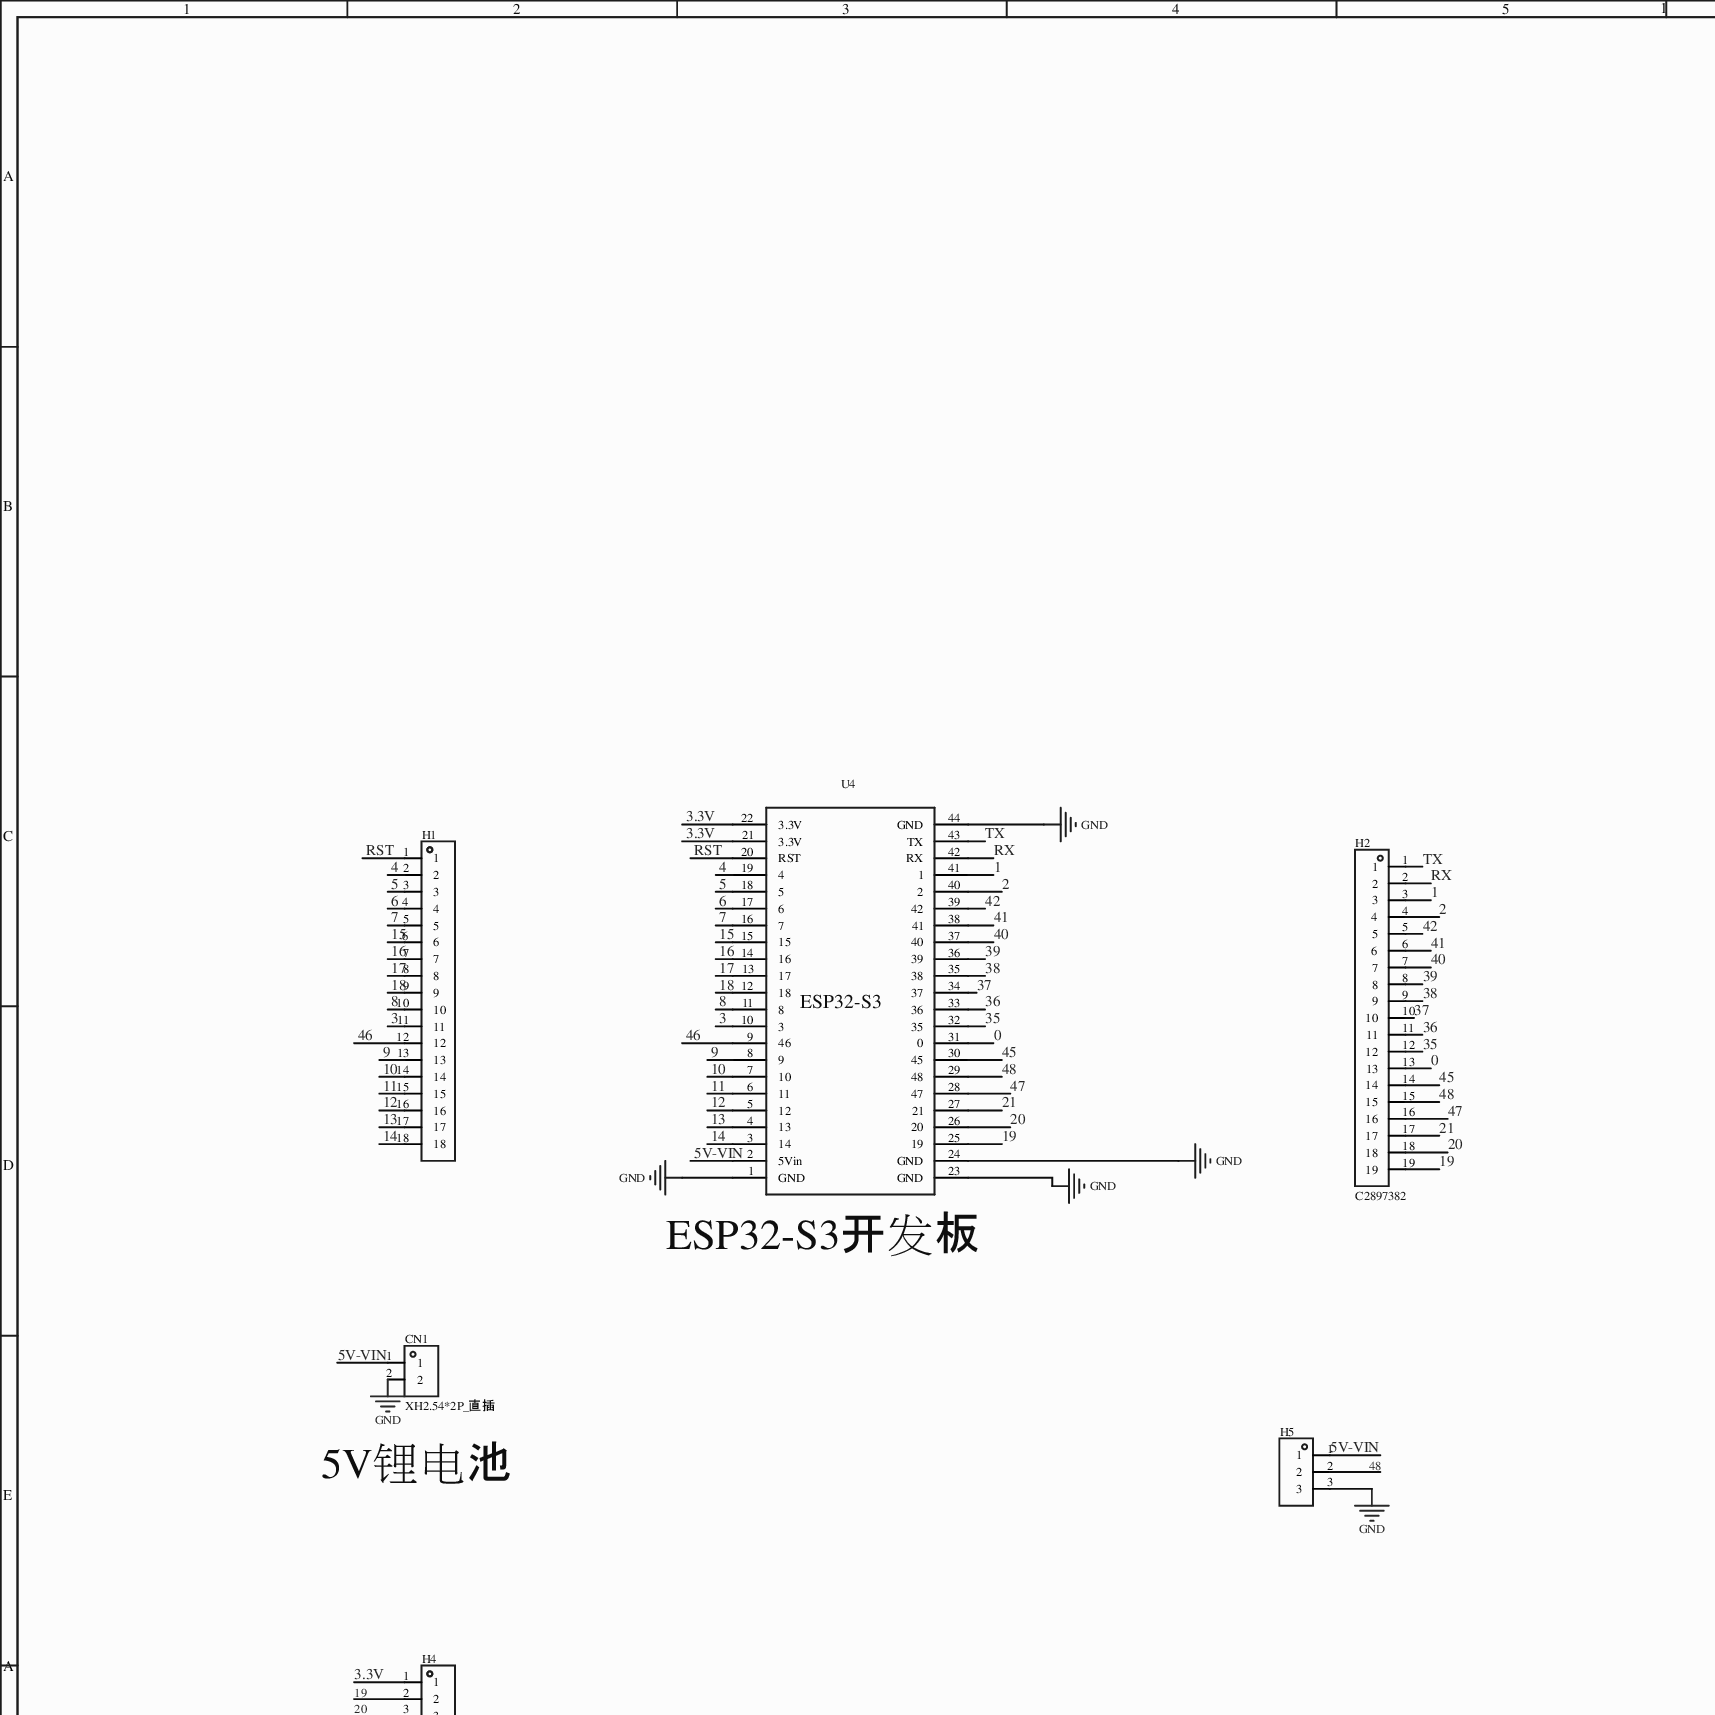
[diagram p0: MISC52029-3.schdoc, top left]
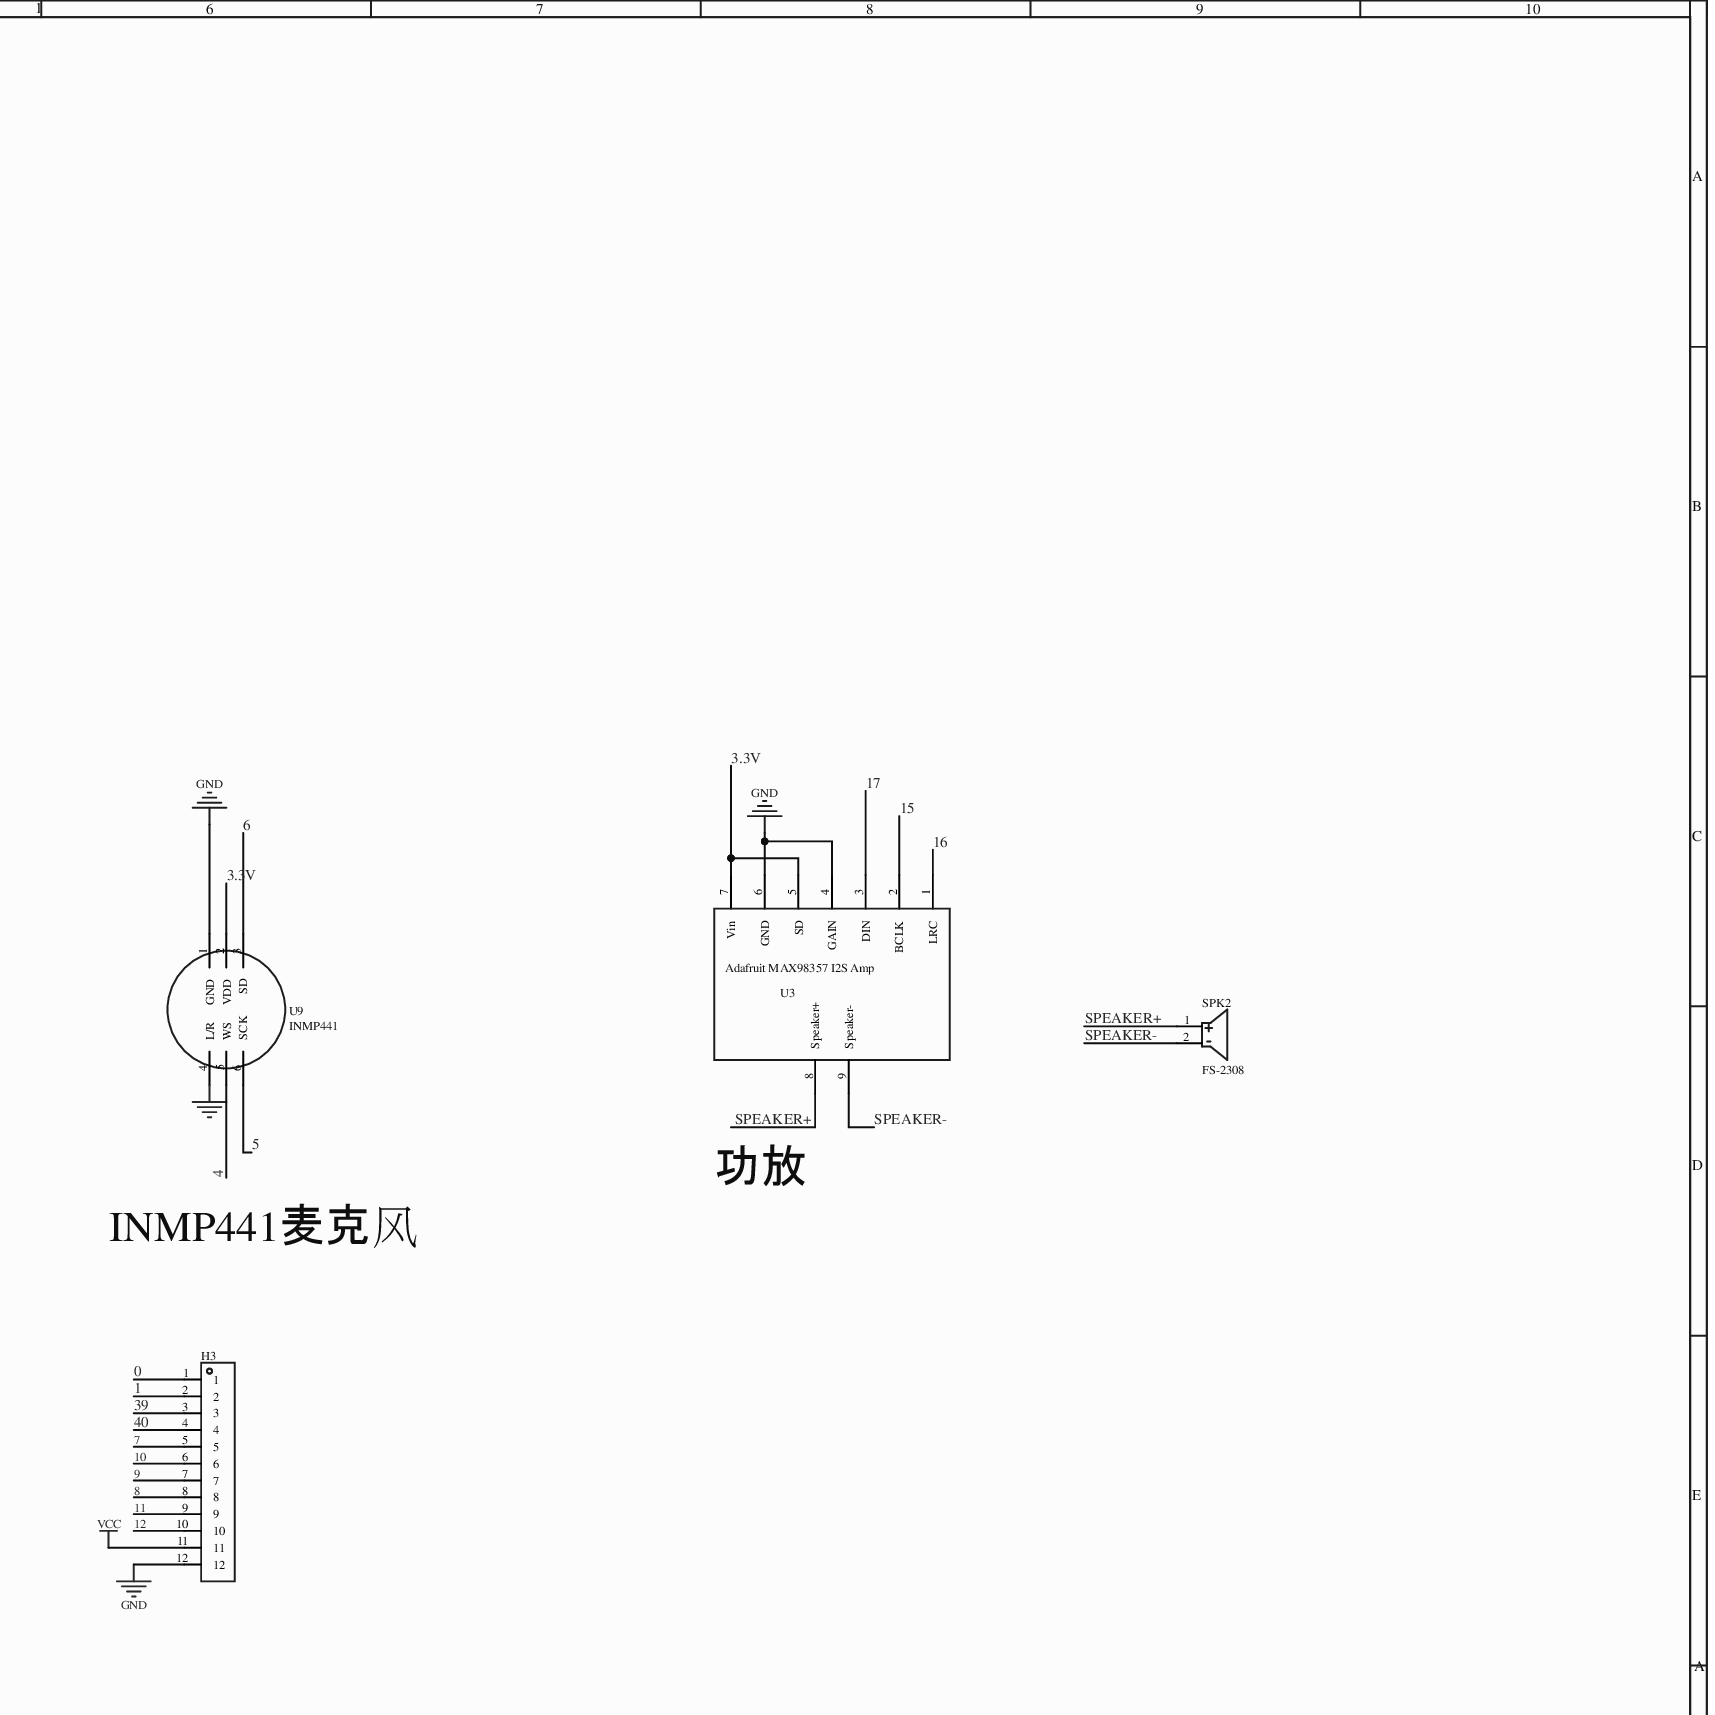
[diagram p1: MISC52029-3.schdoc, top right]
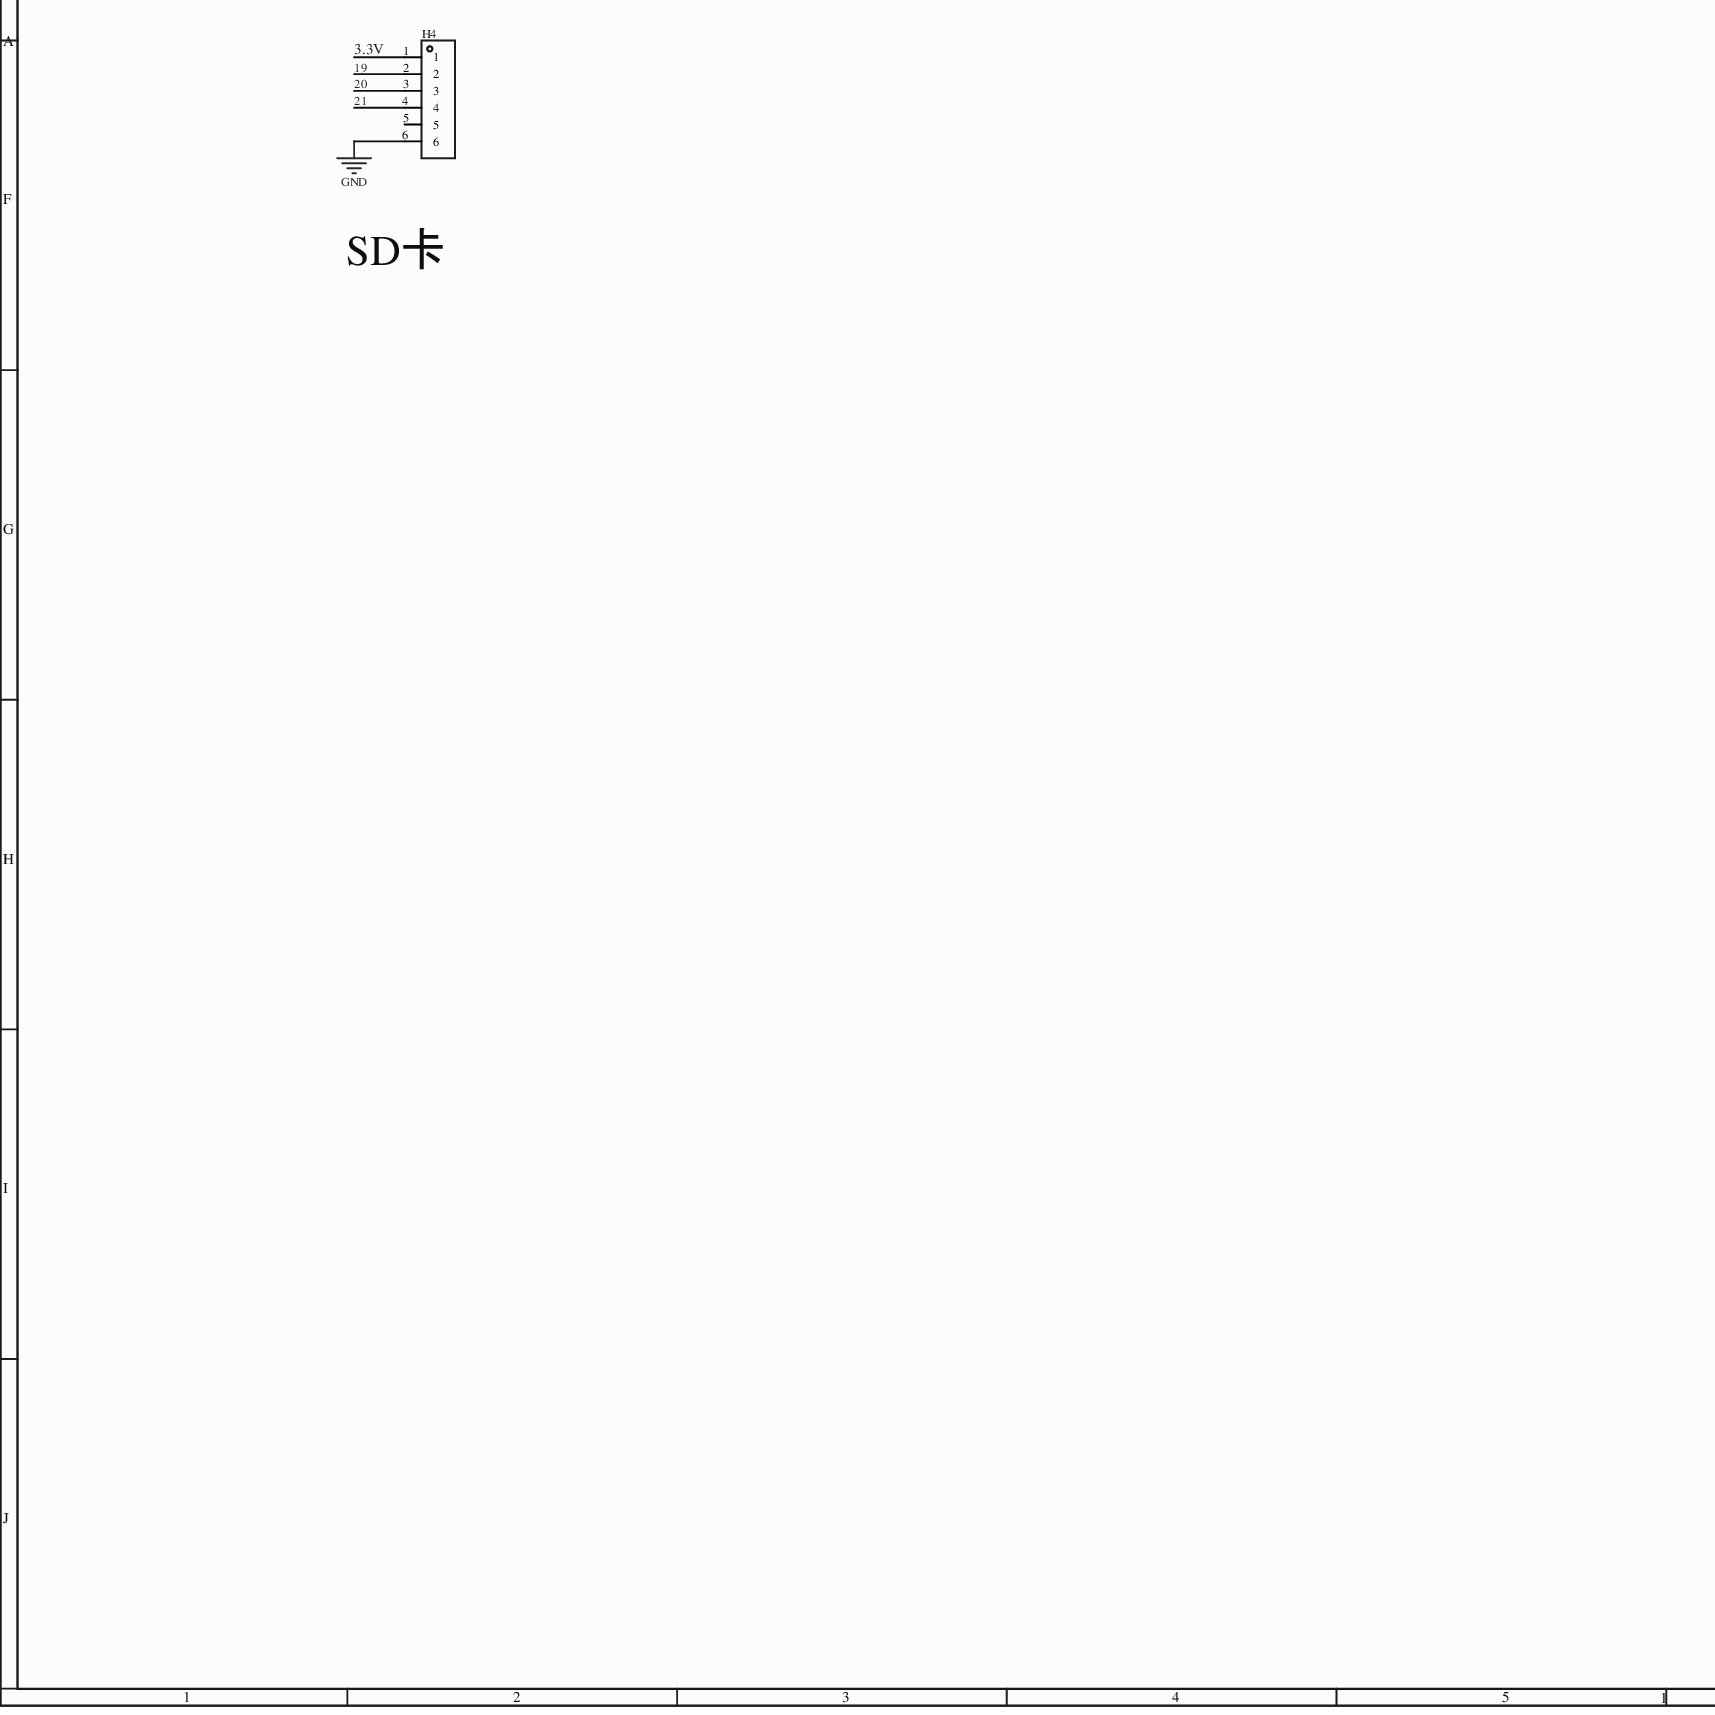
[diagram p2: MISC52029-3.schdoc, bottom left]
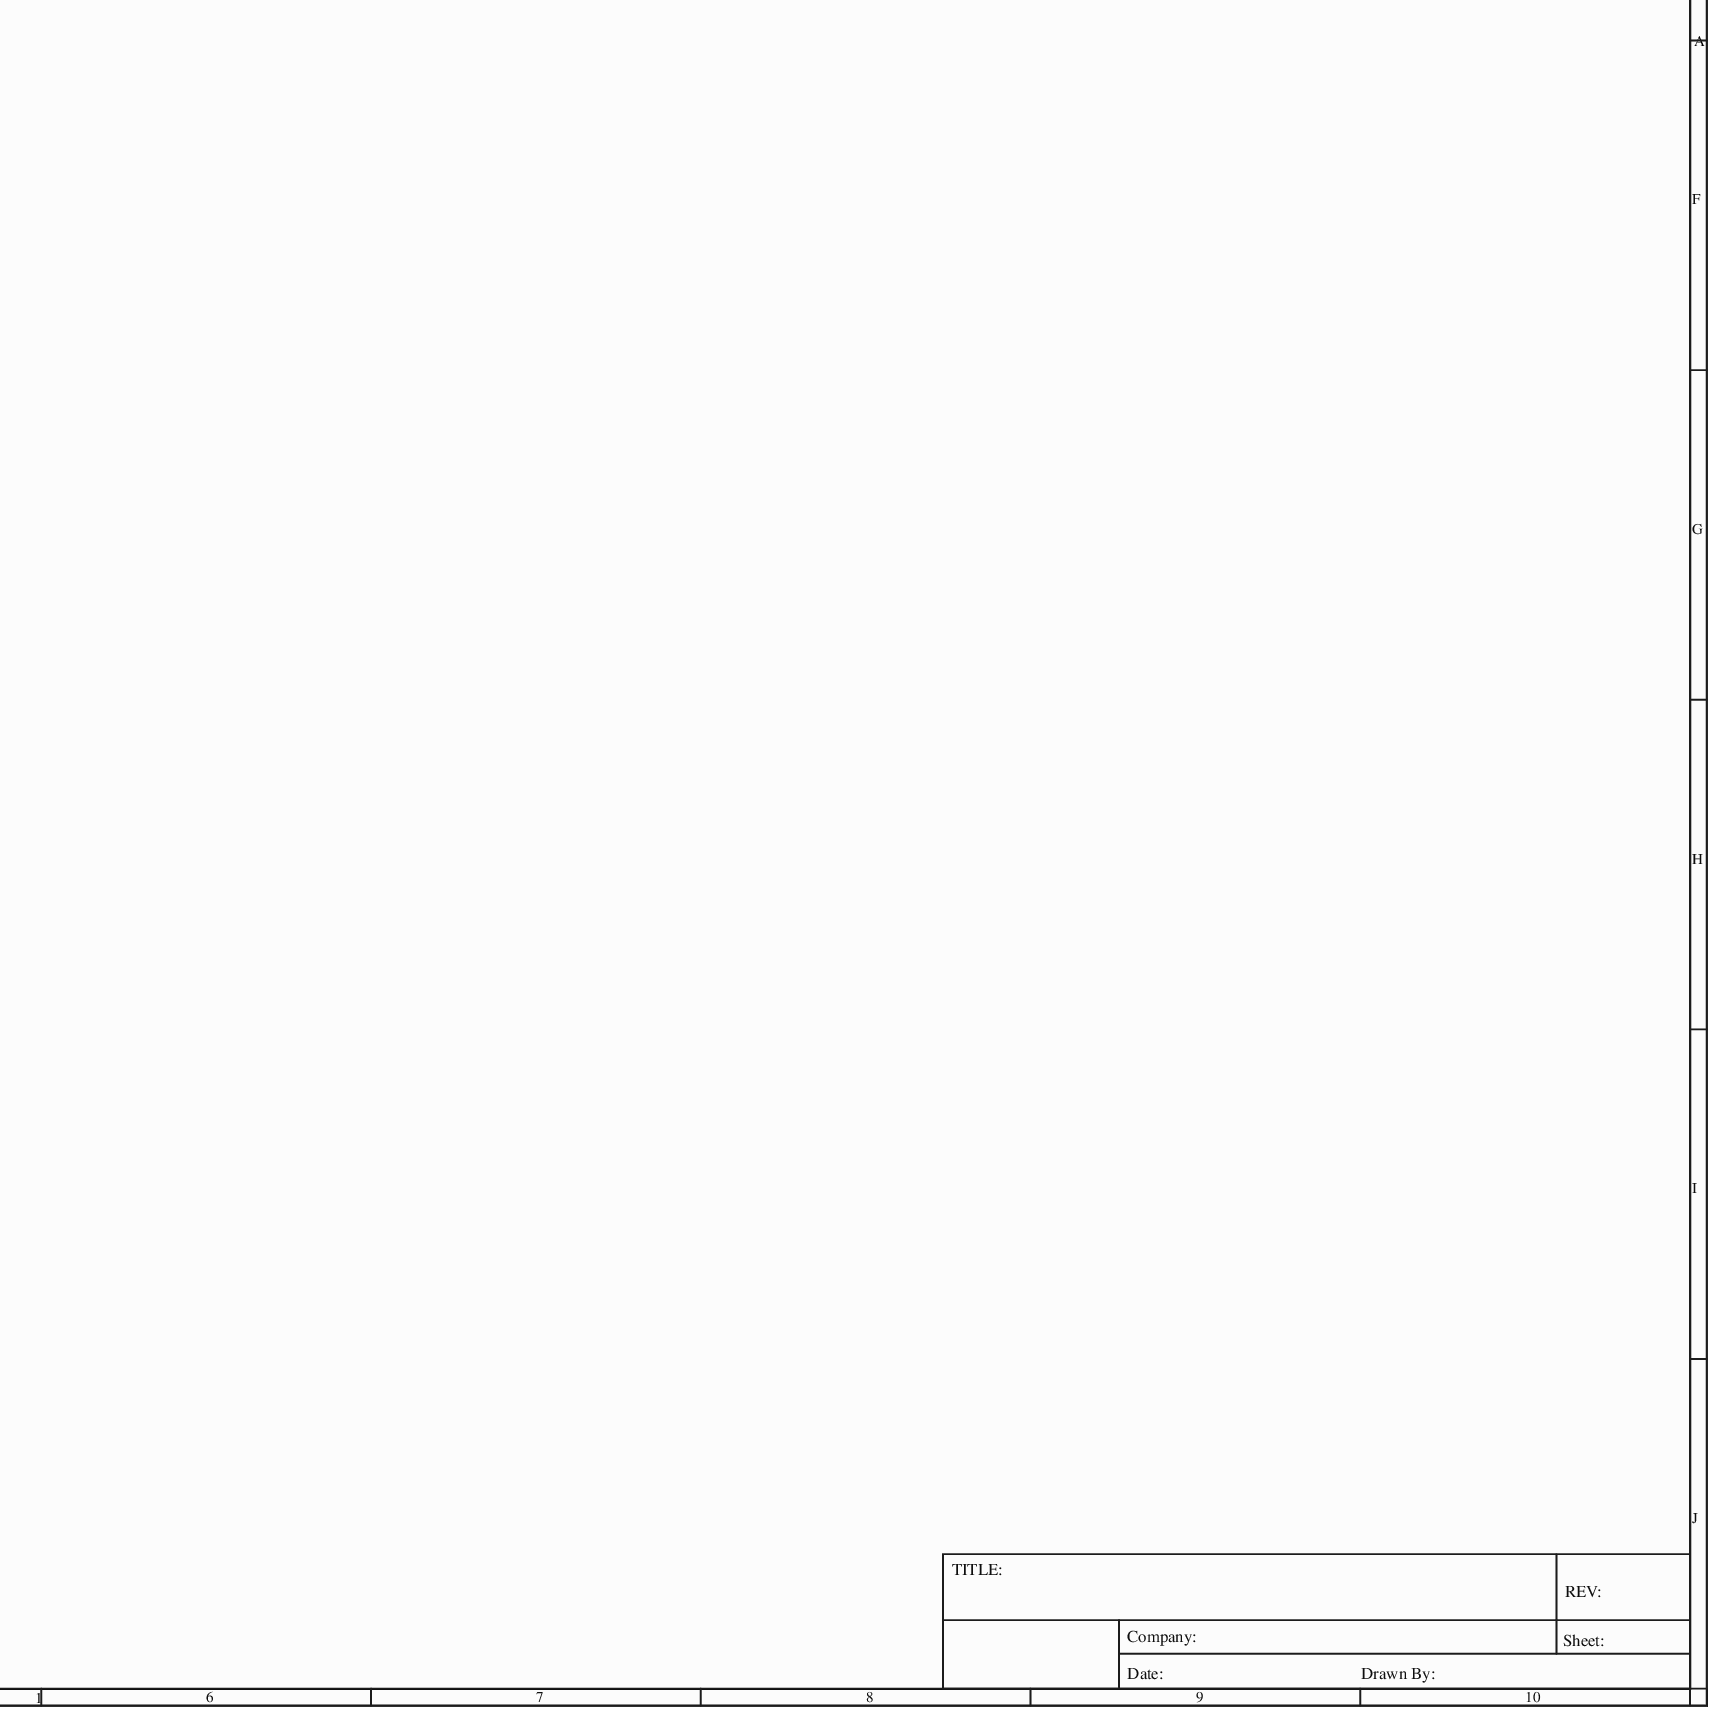
[diagram p3: MISC52029-3.schdoc, bottom right]
# Altium project MISC52029-2.PrjPcb
1 sheet, 10 parts. Net scope: global (net labels, ports and power ports of the same name join across sheets).
Board file: MISC52029.pcbdoc

## Sheet MISC52029-3.schdoc
size 503 x 503 mm; Name: MISC52029; @Project Name: MISC52029; @Page No: 1; @Page Count: 1; @Schematic Name: MISC52029; @Board Name: MISC52029; @Update Date: 2026-05-12; @Create Time: 13:59:00; @Update Time: 16:32:12; @Create Date: 2026-05-12

### Parts
CN1  XH2.54*2P_直插  [CONN-TH_2P-P2.50-XH2.54-2P]
H1  (no value)  [HDR-TH_18P-P2.54-V-F]
H2  C2897382  [HDR-TH_19P-P2.54-V-F]
H3  (no value)  [HDR-TH_12P-P2.54-V-F]
H4  (no value)  [HDR-TH_6P-P2.54-V-F]
H5  (no value)  [HDR-TH_3P-P2.54-V-F]
SPK2  FS-2308  [BEEP-TH_BD23.2-P9.20-D1.0]
U3  Adafruit MAX98357 I2S Amp  [MAX98357 I2S AMP MODULE]
U4  NO  [ESP32S3]  (value not drawn)
U9  INMP441  [INMP441]

### Nets
GND: CN1.2 H3.12 H4.6 H5.3 U3.4(GAIN) U3.6(GND) U4.1(GND) U4.23(GND) U4.24(GND) U4.44(GND) U9.1(GND) U9.4(L/R)
VCC: H3.11
0: H2.13 H3.1 U4.31(0)
1: H2.3 H3.2 U4.41(1)
2: H2.4 U4.40(2)
3: H1.11 U4.10(3)
3.3V: H4.1 U3.5(SD) U3.7(Vin) U4.21(3.3V) U4.22(3.3V) U9.2(VDD)
4: H1.2 U4.19(4) U9.5(WS)
5: H1.3 U4.18(5) U9.6(SCK)
5V-VIN: CN1.1 H5.1 U4.2(5Vin)
6: H1.4 U4.17(6) U9.3(SD)
7: H1.5 H3.5 U4.16(7)
8: H1.10 H3.8 U4.11(8)
9: H1.13 H3.7 U4.8(9)
10: H1.14 H3.6 U4.7(10)
11: H1.15 H3.9 U4.6(11)
12: H1.16 H3.10 U4.5(12)
13: H1.17 U4.4(13)
14: H1.18 U4.3(14)
15: H1.6 U3.2(BCLK) U4.15
16: H1.7 U3.1(LRC) U4.14(16)
17: H1.8 U3.3(DIN) U4.13(17)
18: H1.9 U4.12(18)
19: H2.19 H4.2 U4.25(19)
20: H2.18 H4.3 U4.26(20)
21: H2.17 H4.4 U4.27(21)
35: H2.12 U4.32(35)
36: H2.11 U4.33(36)
37: H2.10 U4.34(37)
38: H2.9 U4.35(38)
39: H2.8 H3.3 U4.36(39)
40: H2.7 H3.4 U4.37(40)
41: H2.6 U4.38(41)
42: H2.5 U4.39(42)
45: H2.14 U4.30(45)
46: H1.12 U4.9(46)
47: H2.16 U4.28(47)
48: H2.15 H5.2 U4.29(48)
RST: H1.1 U4.20(RST)
RX: H2.2 U4.42(RX)
SPEAKER+: SPK2.1 U3.8(Speaker+)
SPEAKER-: SPK2.2 U3.9(Speaker-)
TX: H2.1 U4.43(TX)

Not connected (* = marked no-connect by the designer): H4 5

### Notes on the sheet
- (near U4) ESP32-S3开发板
- INMP441麦克风
- 功放
- (near CN1) 5V锂电池
- SD卡
- 1
- 2
- 3
- 4
- 5
- 6
- 7
- 8
- 9
- 10
- A
- B
- C
- D
- E
- F
- G
- H
- I
- J
- TITLE:
- Company:
- Sheet:
- REV:
- Date:
- Drawn By:

### Library data of the parts
CN1 = XH2.54*2P_直插: AddInBom: yes; ModelId: 325c595e30db4df8abe76612dd40b0fa0819f05c4eef4c71ace90d822a990e87; ModelTransform: 295.275,228.346,0,180,0,0,-0.002,-20.079,-137.795; Symbol: XH2.54*2P_直插; Device: XH2.54*2P_直插; LCSC Part Name: XH2.54*2P_直插; SupplierPart: C9900008615; ManufacturerPart: XH2.54*2P_直插; Supplier Footprint: XH2.54_2P; JLCPCB Part Class: Extended Part; Supplier: LCSC; ConvertToPcb: yes; FootprintName: CONN-TH_2P-P2.50-XH2.54-2P; ModelName: CONN-TH_2P-P2.50-XH2.54-2P
H1 = HDR-F_2.54_1x18P: ConvertToPcb: yes; ModelId: 069cd2213eca4834a2bee4e281fb45db0819f05c4eef4c71ace90d822a990e87; ModelTransform: 1819.681,98.425,0,0,0,0,0,0,-118.11; Symbol: HDR-F_2.54_1x18P; Device: HDR-F_2.54_1x18P; AddInBom: yes; SupplierPart: C2897381; Supplier Footprint: 插件; FootprintName: HDR-TH_18P-P2.54-V-F; ModelName: HDR-TH_18P-P2.54-V-F
H2 = HDR-F_2.54_1x19P: ConvertToPcb: yes; ModelId: 131ee080550a465daf9368d356f53fe90819f05c4eef4c71ace90d822a990e87; ModelName: HDR-TH_19P-P2.54-F-LI-1X19P; ModelTransform: 1919.68128,95.6691,0,0,0,0,0,0,-125.984; Symbol: HDR-F_2.54_1x19P; Device: HDR-F_2.54_1x19P; AddInBom: yes; Supplier Footprint: 插件; ManufacturerPart: C2897382; FootprintName: HDR-TH_19P-P2.54-V-F
H3 = HDR-F_2.54_1x12P: ConvertToPcb: yes; ModelId: a8b4b2347edc4eeab5667ae97bf18e170819f05c4eef4c71ace90d822a990e87; ModelName: HDR-TH_12P-P2.54-F-LI-1X12P; ModelTransform: 1215.74568,98.425,0,0,0,0,0,0,-129.921; Symbol: HDR-F_2.54_1x12P; Device: HDR-F_2.54_1x12P; AddInBom: yes; SupplierPart: C2905419; Supplier Footprint: 插件; FootprintName: HDR-TH_12P-P2.54-V-F
H4 = HDR-F_2.54_1x6P: Symbol: Header-Female-2.54_1x6; ConvertToPcb: yes; ModelId: 0f5bcf94dcda47d085f24cdca1696fe90819f05c4eef4c71ace90d822a990e87; ModelTransform: 619.684,94.488,0,0,0,0,0,0,-125.984; Device: HDR-F_2.54_1x6P; AddInBom: yes; SupplierPart: C40877; Supplier Footprint: 插件; FootprintName: HDR-TH_6P-P2.54-V-F; ModelName: HDR-TH_6P-P2.54-V-F
H5 = HDR-F_2.54_1x3P: Symbol: PM254V-11-03-H85; ConvertToPcb: yes; ModelId: f3b3cc5aae9641bf9e56fc160cef875b0819f05c4eef4c71ace90d822a990e87; ModelName: HDR2.54-F-LI-1X3P; ModelTransform: 299.9994,100,0,0,0,0,0,0,-118.11; Device: HDR-F_2.54_1x3P; AddInBom: yes; SupplierPart: C541850; Supplier Footprint: 插件; FootprintName: HDR-TH_3P-P2.54-V-F
SPK2 = FS-2308: Manufacturer: FUET(福声科技); Add into BOM: yes; ModelId: f2de6d3d53f440b38eb7d42236cfa69c; ModelTransform: 905.51,905.51,0,90,0,0,0,0,-118.11; Symbol: FS-2308; Device: FS-2308; LCSC Part Name: 喇叭23MM-8.0H 8Ω1W 插针; SupplierPart: C482322; ManufacturerPart: FS-2308; Supplier Footprint: -; JLCPCB Part Class: 扩展库; Datasheet: https://atta.szlcsc.com/upload/public/pdf/source/20200113/C482322_D09CD61BAFBB8D4AD64070E01BFD18FF.pdf; Supplier: LCSC; ConvertToPcb: yes; FootprintName: BEEP-TH_BD23.2-P9.20-D1.0; ModelName: BEEP-TH_BD23.2-P9.20-D1.0
U3 = Adafruit MAX98357 I2S Amp: Convert to PCB: yes; Origin Footprint: MAX98357 I2S AMP MODULE; Device: Adafruit MAX98357 I2S Amp; Symbol: Adafruit MAX98357 I2S Amp; Manufacturer Part: Adafruit MAX98357 I2S Amp; Add into BOM: yes; FootprintName: MAX98357 I2S AMP MODULE
U4 = NO: Convert to PCB: yes; Origin Footprint: ESP32S3; Device: NO; Symbol: NO; Add into BOM: yes; FootprintName: ESP32S3
U9 = INMP441: Convert to PCB: yes; Origin Footprint: INMP441; Device: INMP441; Symbol: INMP441; Add into BOM: yes; FootprintName: INMP441